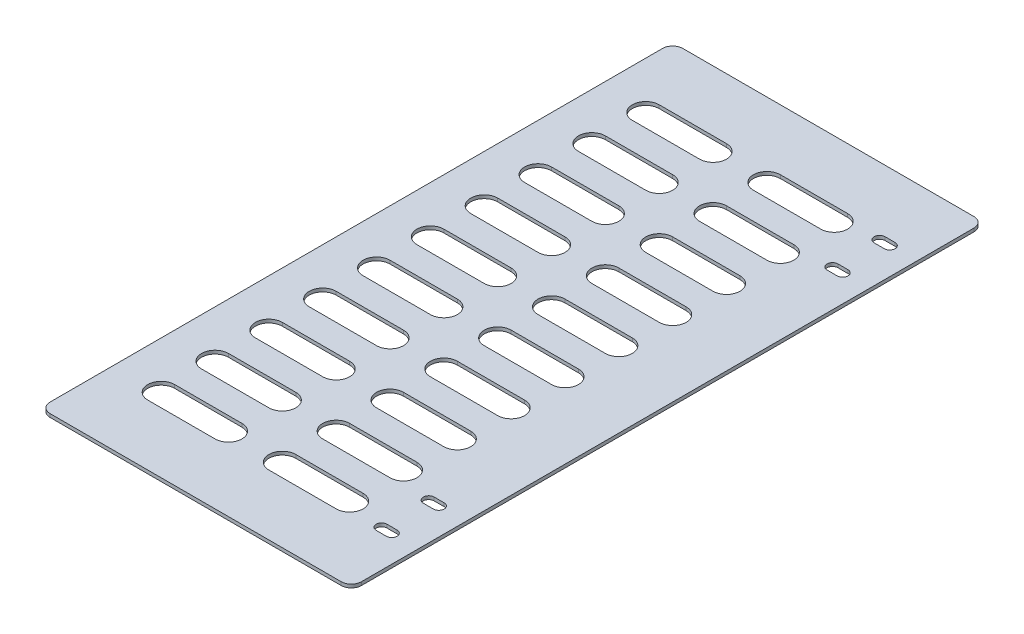
SolidWorks part; units mm, degrees
material "Thornel Mat VMA"
ref_plane "前视基准面" through (0, 0, 0) normal (0, 0, 1) x (1, 0, 0)
ref_plane "上视基准面" through (0, 0, 0) normal (0, 1, 0) x (1, 0, 0)
ref_plane "右视基准面" through (0, 0, 0) normal (1, 0, 0) x (0, 0, -1)
other "Configuration Table"
sketch "草图1" plane through (0, 0, 0) normal (0, 1, 0) x (1, 0, 0)
  line L1 (-46.25, -94) -> (46.25, -94)
  line L2 (-46.25, -94) -> (-46.25, 94)
  line L3 (-46.25, 94) -> (46.25, 94)
  line L4 (46.25, -94) -> (46.25, 94)
  line L5 (-46.25, -94) -> (46.25, 94) construction
  line L6 (-46.25, 94) -> (46.25, -94) construction
  point P0 (0, 0)
  dimension "D1" = 188
  dimension "D2" = 92.5
extrude "凸台-拉伸1" add sketch "草图1" along normal blind 1
fillet "圆角1" radius 3 4 edges at (-46.25, 0.5, -94) (46.25, 0.5, -94) (46.25, 0.5, 94) (-46.25, 0.5, 94)
sketch "草图3" plane through (0, 1, 0) normal (0, 1, 0) x (1, 0, 0)
  line L0 (35.25, 94) -> (35.25, 74) construction
  line L1 (43.25, 94) -> (-43.25, 94) construction
  line L2 (35.25, 74) -> (35.25, 60) construction
  line L3 (35.25, 60) -> (38.25, 60) construction
  line L4 (35.25, 61.6) -> (38.25, 61.6)
  line L5 (35.25, 58.4) -> (38.25, 58.4)
  line L6 (35.25, 74) -> (38.25, 74) construction
  line L7 (35.25, 75.6) -> (38.25, 75.6)
  line L8 (35.25, 72.4) -> (38.25, 72.4)
  line L9 (46.25, -91) -> (46.25, 91) construction
  line L10 (0, 0) -> (141.8819, 0) construction
  line L11 (35.25, -60) -> (38.25, -60) construction
  line L12 (35.25, -61.6) -> (38.25, -61.6)
  line L13 (35.25, -58.4) -> (38.25, -58.4)
  line L14 (35.25, -74) -> (38.25, -74) construction
  line L15 (35.25, -75.6) -> (38.25, -75.6)
  line L16 (35.25, -72.4) -> (38.25, -72.4)
  line L17 (35.25, -74) -> (35.25, -60) construction
  line L18 (35.25, -94) -> (35.25, -74) construction
  arc A0 (35.25, 61.6) -> (35.25, 58.4) centre (35.25, 60) ccw
  arc A1 (38.25, 58.4) -> (38.25, 61.6) centre (38.25, 60) ccw
  arc A2 (35.25, 75.6) -> (35.25, 72.4) centre (35.25, 74) ccw
  arc A3 (38.25, 72.4) -> (38.25, 75.6) centre (38.25, 74) ccw
  arc A4 (35.25, -61.6) -> (35.25, -58.4) centre (35.25, -60) cw
  arc A5 (38.25, -58.4) -> (38.25, -61.6) centre (38.25, -60) cw
  arc A6 (35.25, -75.6) -> (35.25, -72.4) centre (35.25, -74) cw
  arc A7 (38.25, -72.4) -> (38.25, -75.6) centre (38.25, -74) cw
  point P5 (36.75, 60)
  point P11 (36.75, 74)
  point P24 (36.75, -60)
  point P31 (36.75, -74)
  dimension "D2" = 1.6
  dimension "D1" = 3
  dimension "D3" = 20
  dimension "D4" = 14
  dimension "D5" = 11
extrude "切除-拉伸2" cut sketch "草图3" against normal blind 10
sketch "草图4" plane through (0, 1, 0) normal (0, 1, 0) x (1, 0, 0)
  line L0 (-32.25, 8) -> (-12.25, 8) construction
  line L1 (-32.25, 12) -> (-12.25, 12)
  line L2 (-32.25, 4) -> (-12.25, 4)
  line L3 (3.75, 8) -> (23.75, 8) construction
  line L4 (3.75, 12) -> (23.75, 12)
  line L5 (3.75, 4) -> (23.75, 4)
  line L6 (3.75, -72) -> (23.75, -72) construction
  line L7 (-46.25, 91) -> (-46.25, -91) construction
  line L8 (0, 0) -> (108.9091, 0) construction
  line L9 (-32.25, 24) -> (-12.25, 24) construction
  line L10 (-32.25, 28) -> (-12.25, 28)
  line L11 (-32.25, 20) -> (-12.25, 20)
  line L12 (3.75, 24) -> (23.75, 24) construction
  line L13 (3.75, 28) -> (23.75, 28)
  line L14 (3.75, 20) -> (23.75, 20)
  line L15 (-32.25, 40) -> (-12.25, 40) construction
  line L16 (-32.25, 44) -> (-12.25, 44)
  line L17 (-32.25, 36) -> (-12.25, 36)
  line L18 (3.75, 40) -> (23.75, 40) construction
  line L19 (3.75, 44) -> (23.75, 44)
  line L20 (3.75, 36) -> (23.75, 36)
  line L21 (-32.25, 56) -> (-12.25, 56) construction
  line L22 (-32.25, 60) -> (-12.25, 60)
  line L23 (-32.25, 52) -> (-12.25, 52)
  line L24 (3.75, 56) -> (23.75, 56) construction
  line L25 (3.75, 60) -> (23.75, 60)
  line L26 (3.75, 52) -> (23.75, 52)
  line L27 (-32.25, 72) -> (-12.25, 72) construction
  line L28 (-32.25, 76) -> (-12.25, 76)
  line L29 (-32.25, 68) -> (-12.25, 68)
  line L30 (3.75, 72) -> (23.75, 72) construction
  line L31 (3.75, 76) -> (23.75, 76)
  line L32 (3.75, 68) -> (23.75, 68)
  line L33 (3.75, -76) -> (23.75, -76)
  line L34 (3.75, -68) -> (23.75, -68)
  line L35 (-32.25, -72) -> (-12.25, -72) construction
  line L36 (-32.25, -76) -> (-12.25, -76)
  line L37 (-32.25, -68) -> (-12.25, -68)
  line L38 (3.75, -56) -> (23.75, -56) construction
  line L39 (3.75, -60) -> (23.75, -60)
  line L40 (3.75, -52) -> (23.75, -52)
  line L41 (-32.25, -56) -> (-12.25, -56) construction
  line L42 (-32.25, -60) -> (-12.25, -60)
  line L43 (-32.25, -52) -> (-12.25, -52)
  line L44 (3.75, -40) -> (23.75, -40) construction
  line L45 (3.75, -44) -> (23.75, -44)
  line L46 (3.75, -36) -> (23.75, -36)
  line L47 (-32.25, -40) -> (-12.25, -40) construction
  line L48 (-32.25, -44) -> (-12.25, -44)
  line L49 (-32.25, -36) -> (-12.25, -36)
  line L50 (3.75, -24) -> (23.75, -24) construction
  line L51 (3.75, -28) -> (23.75, -28)
  line L52 (3.75, -20) -> (23.75, -20)
  line L53 (-32.25, -24) -> (-12.25, -24) construction
  line L54 (-32.25, -28) -> (-12.25, -28)
  line L55 (-32.25, -20) -> (-12.25, -20)
  line L56 (3.75, -8) -> (23.75, -8) construction
  line L57 (3.75, -12) -> (23.75, -12)
  line L58 (3.75, -4) -> (23.75, -4)
  line L59 (-32.25, -8) -> (-12.25, -8) construction
  line L60 (-32.25, -12) -> (-12.25, -12)
  line L61 (-32.25, -4) -> (-12.25, -4)
  arc A0 (-32.25, 12) -> (-32.25, 4) centre (-32.25, 8) ccw
  arc A1 (-12.25, 4) -> (-12.25, 12) centre (-12.25, 8) ccw
  arc A2 (3.75, 12) -> (3.75, 4) centre (3.75, 8) ccw
  arc A3 (23.75, 4) -> (23.75, 12) centre (23.75, 8) ccw
  arc A4 (-32.25, 28) -> (-32.25, 20) centre (-32.25, 24) ccw
  arc A5 (-12.25, 20) -> (-12.25, 28) centre (-12.25, 24) ccw
  arc A6 (3.75, 28) -> (3.75, 20) centre (3.75, 24) ccw
  arc A7 (23.75, 20) -> (23.75, 28) centre (23.75, 24) ccw
  arc A8 (-32.25, 44) -> (-32.25, 36) centre (-32.25, 40) ccw
  arc A9 (-12.25, 36) -> (-12.25, 44) centre (-12.25, 40) ccw
  arc A10 (3.75, 44) -> (3.75, 36) centre (3.75, 40) ccw
  arc A11 (23.75, 36) -> (23.75, 44) centre (23.75, 40) ccw
  arc A12 (-32.25, 60) -> (-32.25, 52) centre (-32.25, 56) ccw
  arc A13 (-12.25, 52) -> (-12.25, 60) centre (-12.25, 56) ccw
  arc A14 (3.75, 60) -> (3.75, 52) centre (3.75, 56) ccw
  arc A15 (23.75, 52) -> (23.75, 60) centre (23.75, 56) ccw
  arc A16 (-32.25, 76) -> (-32.25, 68) centre (-32.25, 72) ccw
  arc A17 (-12.25, 68) -> (-12.25, 76) centre (-12.25, 72) ccw
  arc A18 (3.75, 76) -> (3.75, 68) centre (3.75, 72) ccw
  arc A19 (23.75, 68) -> (23.75, 76) centre (23.75, 72) ccw
  arc A20 (3.75, -76) -> (3.75, -68) centre (3.75, -72) cw
  arc A21 (23.75, -68) -> (23.75, -76) centre (23.75, -72) cw
  arc A22 (-32.25, -76) -> (-32.25, -68) centre (-32.25, -72) cw
  arc A23 (-12.25, -68) -> (-12.25, -76) centre (-12.25, -72) cw
  arc A24 (3.75, -60) -> (3.75, -52) centre (3.75, -56) cw
  arc A25 (23.75, -52) -> (23.75, -60) centre (23.75, -56) cw
  arc A26 (-32.25, -60) -> (-32.25, -52) centre (-32.25, -56) cw
  arc A27 (-12.25, -52) -> (-12.25, -60) centre (-12.25, -56) cw
  arc A28 (3.75, -44) -> (3.75, -36) centre (3.75, -40) cw
  arc A29 (23.75, -36) -> (23.75, -44) centre (23.75, -40) cw
  arc A30 (-32.25, -44) -> (-32.25, -36) centre (-32.25, -40) cw
  arc A31 (-12.25, -36) -> (-12.25, -44) centre (-12.25, -40) cw
  arc A32 (3.75, -28) -> (3.75, -20) centre (3.75, -24) cw
  arc A33 (23.75, -20) -> (23.75, -28) centre (23.75, -24) cw
  arc A34 (-32.25, -28) -> (-32.25, -20) centre (-32.25, -24) cw
  arc A35 (-12.25, -20) -> (-12.25, -28) centre (-12.25, -24) cw
  arc A36 (3.75, -12) -> (3.75, -4) centre (3.75, -8) cw
  arc A37 (23.75, -4) -> (23.75, -12) centre (23.75, -8) cw
  arc A38 (-32.25, -12) -> (-32.25, -4) centre (-32.25, -8) cw
  arc A39 (-12.25, -4) -> (-12.25, -12) centre (-12.25, -8) cw
  point P2 (-22.25, 8)
  point P7 (13.75, 8)
  point P20 (13.75, -72)
  point P23 (-22.25, 24)
  point P28 (13.75, 24)
  point P37 (-22.25, 40)
  point P42 (13.75, 40)
  point P51 (-22.25, 56)
  point P56 (13.75, 56)
  point P65 (-22.25, 72)
  point P70 (13.75, 72)
  point P83 (-22.25, -72)
  point P90 (13.75, -56)
  point P97 (-22.25, -56)
  point P104 (13.75, -40)
  point P111 (-22.25, -40)
  point P118 (13.75, -24)
  point P125 (-22.25, -24)
  point P132 (13.75, -8)
  point P139 (-22.25, -8)
  dimension "D2" = 4
  dimension "D4" = 4
  dimension "D1" = 20
  dimension "D3" = 20
  dimension "D5" = 8
  dimension "D6" = 14
  dimension "D7" = 16
  dimension "D9" = 16
  dimension "D8" = 5
extrude "切除-拉伸3" cut sketch "草图4" against normal blind 10
